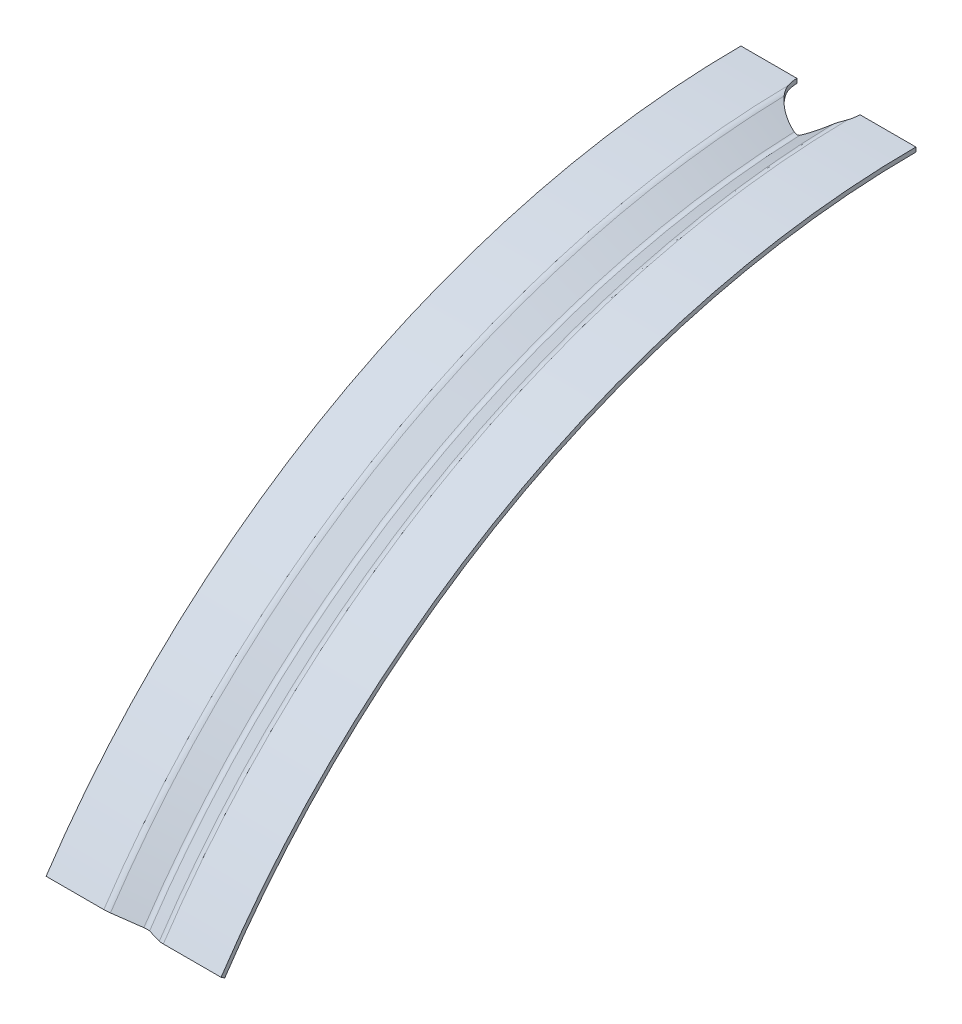
SolidWorks part; units mm, degrees
material "普通碳钢"
ref_plane "Front Plane" through (0, 0, 0) normal (0, 0, 1) x (1, 0, 0)
ref_plane "Top Plane" through (0, 0, 0) normal (0, 1, 0) x (1, 0, 0)
ref_plane "Right Plane" through (0, 0, 0) normal (1, 0, 0) x (0, 0, -1)
sketch "Sketch1" plane through (0, 0, 0) normal (0, 0, 1) x (1, 0, 0)
  line L0 (-102.059, 0) -> (82.9683, 0) construction
  line L1 (0, 78.4311) -> (0, -36.3795) construction
  line L2 (-158.75, 20.7) -> (-53.975, 20.7)
  line L3 (-158.75, 20.7) -> (-158.75, 12.7)
  line L4 (-158.75, 12.7) -> (-53.975, 12.7)
  line L5 (65.1452, 3.175) -> (36.467, 3.175) construction
  line L6 (-53.975, 63.7326) -> (-53.975, -14.1942) construction
  line L7 (-65.1452, 3.175) -> (-36.467, 3.175) construction
  line L8 (-44.3314, 17.8081) -> (-5.2414, -7.9532)
  line L9 (-48.7336, 11.1282) -> (-9.6436, -14.6331)
  line L10 (48.7336, 11.1282) -> (9.6436, -14.6331)
  line L11 (44.3314, 17.8081) -> (5.2414, -7.9532)
  line L12 (158.75, 12.7) -> (53.975, 12.7)
  line L13 (158.75, 20.7) -> (158.75, 12.7)
  line L14 (158.75, 20.7) -> (53.975, 20.7)
  arc A0 (-5.2414, -7.9532) -> (5.2414, -7.9532) centre (0, 0) ccw
  arc A1 (-48.7336, 11.1282) -> (-53.975, 12.7) centre (-53.975, 3.175) ccw
  arc A2 (-44.3314, 17.8081) -> (-53.975, 20.7) centre (-53.975, 3.175) ccw
  arc A3 (-9.6436, -14.6331) -> (9.6436, -14.6331) centre (0, 0) ccw
  arc A4 (-17.5244, 0.1416) -> (-17.525, 0) centre (0, 0) ccw
  circle A5 centre (0, 0) radius 17.525 construction
  arc A6 (17.5244, 0.1416) -> (17.525, 0) centre (0, 0) cw
  circle A7 centre (0, 0) radius 9.525 construction
  arc A8 (44.3314, 17.8081) -> (53.975, 20.7) centre (53.975, 3.175) cw
  arc A9 (48.7336, 11.1282) -> (53.975, 12.7) centre (53.975, 3.175) cw
  point P22 (17.525, 0)
  point P30 (9.1088, 2.7848)
  dimension "D1" = 19.05
  dimension "D8" = 8
  dimension "D2" = 8
  dimension "D3" = 12.7
  dimension "D5" = 158.75
  dimension "D6" = 53.975
  dimension "D7" = 9.525
sketch "Sketch2" plane through (0, 0, 0) normal (1, 0, 0) x (0, 0, -1)
  line L1 (393.6282, 20.7) -> (-391.0134, 20.7) construction
  line L2 (0, -1495.425) -> (0, 20.7) construction
  line L3 (0, 20.7) -> (-1260.9943, -653.6837) construction
  arc A0 (0, 20.7) -> (-1260.9943, -653.6837) centre (0, -1495.425) ccw
  dimension "D2" = 20.7
  dimension "D3" = 1516.125
  dimension "D4" = 1430
sweep "Sweep1" add profiles "Sketch1" path "Sketch2"
sketch "Sketch3" plane through (0, 0, 0) normal (0, 1, 0) x (1, 0, 0)
  circle A0 centre (0, 0) radius 57.15
  dimension "D1" = 114.3
extrude "Cut-Extrude1" cut sketch "Sketch3" against normal mid plane 100
